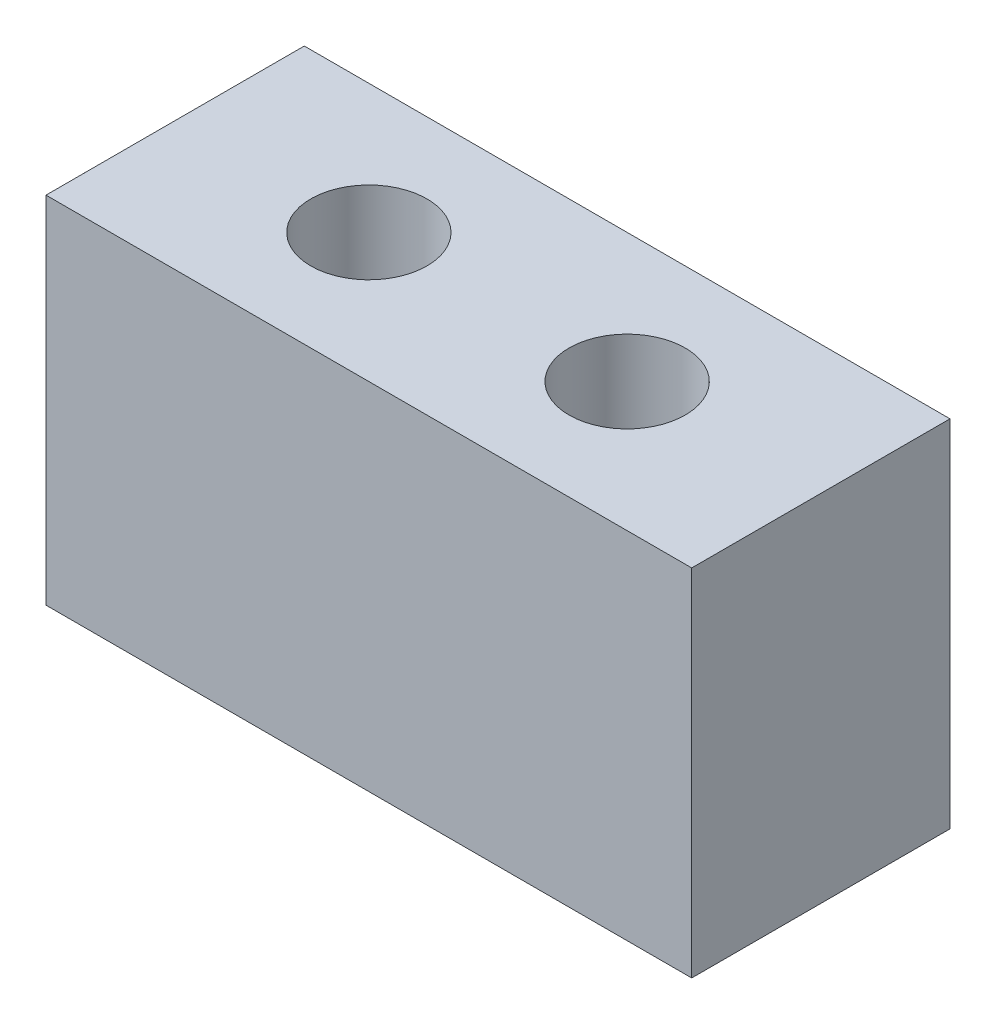
from build123d import *

# Parameters (mm, degrees)
SKETCH1_W           = 100
SKETCH1_H           = 40
SKETCH1_R           = 5.5
BOSS_EXTRUDE1_DEPTH = 55
SKETCH2_R           = 9
CUT_EXTRUDE1_DEPTH  = 20


with BuildPart() as part:
    # Sketch1 → Boss-Extrude1 (new body)
    with BuildSketch(Plane(origin=(0, 0, 0), x_dir=(1, 0, 0), z_dir=(0, 1, 0))):
        Rectangle(SKETCH1_W, SKETCH1_H)
        with Locations(Location((-20, 0, 0), (0, 0, 270))):
            Circle(SKETCH1_R, mode=Mode.SUBTRACT)
        with Locations(Location((20, 0, 0), (0, 0, 270))):
            Circle(SKETCH1_R, mode=Mode.SUBTRACT)
    extrude(amount=BOSS_EXTRUDE1_DEPTH)

    # Sketch2 → Cut-Extrude1 (cut)
    with BuildSketch(Plane(origin=(0, 55, 0), x_dir=(1, 0, 0), z_dir=(0, 1, 0))):
        with Locations(Location((20, 0, 0), (0, 0, 270))):
            Circle(SKETCH2_R)
        with Locations(Location((-20, 0, 0), (0, 0, 270))):
            Circle(SKETCH2_R)
    extrude(amount=-CUT_EXTRUDE1_DEPTH, mode=Mode.SUBTRACT)


solid = part.part
